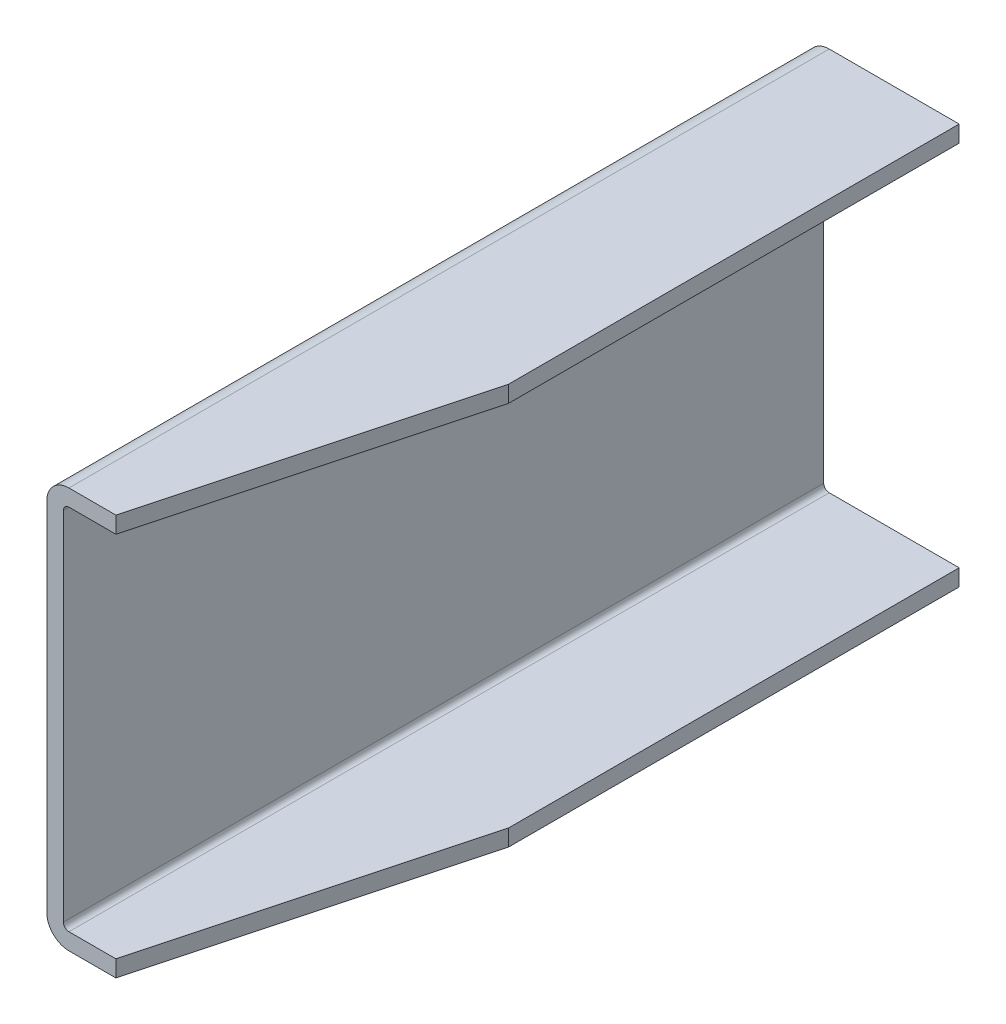
from build123d import *

# Parameters (mm, degrees)
EXTRUDE_1_DEPTH     = 275
CUT_EXTRUDE_1_DEPTH = 275


with BuildPart() as part:
    # 草图1 → 凸台-拉伸1 (new body)
    with BuildSketch(Plane.XY):
        with BuildLine():
            Line((0, 0), (-47, 0))
            ThreePointArc((-47, 0), (-52.656854249, -2.343145751), (-55, -8))
            Line((-55, -8), (-55, -137))
            ThreePointArc((-55, -137), (-52.656854249, -142.656854249), (-47, -145))
            Line((-47, -145), (0, -145))
            Line((0, -145), (0, -139))
            Line((0, -139), (-47, -139))
            ThreePointArc((-47, -139), (-48.414213562, -138.414213562), (-49, -137))
            Line((-49, -137), (-49, -8))
            ThreePointArc((-49, -8), (-48.414213562, -6.585786438), (-47, -6))
            Line((-47, -6), (0, -6))
            Line((0, -6), (0, 0))
        make_face()
    extrude(amount=EXTRUDE_1_DEPTH)

    # 草图2 → 切除-拉伸1 (cut)
    with BuildSketch(Plane(origin=(0, 0, 0), x_dir=(1, 0, 0), z_dir=(0, 1, 0))):
        Polygon((0, -163), (-30, -275), (0, -275), align=None)
    extrude(amount=-CUT_EXTRUDE_1_DEPTH, mode=Mode.SUBTRACT)


solid = part.part
